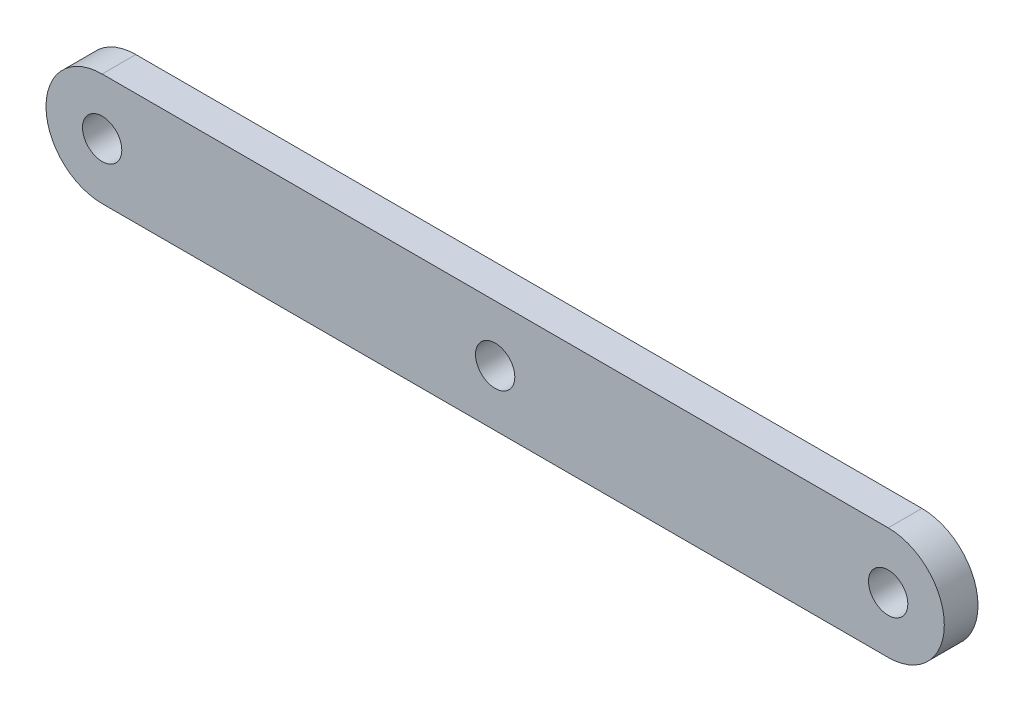
SolidWorks part; units mm, degrees
ref_plane "Front Plane" through (0, 0, 0) normal (0, 0, 1) x (1, 0, 0)
ref_plane "Top Plane" through (0, 0, 0) normal (0, 1, 0) x (1, 0, 0)
ref_plane "Right Plane" through (0, 0, 0) normal (1, 0, 0) x (0, 0, -1)
sketch "Sketch1" plane through (0, 0, 0) normal (0, 0, 1) x (1, 0, 0)
  line L0 (55, 0) -> (-55, 0) construction
  line L1 (0, 10) -> (140, 10)
  line L2 (0, 0) -> (158.2009, 0) construction
  line L3 (0, -10) -> (140, -10)
  arc A0 (0, 10) -> (0, -10) centre (0, 0) ccw
  arc A1 (140, -10) -> (140, 10) centre (140, 0) ccw
  dimension "D1" = 140
  dimension "D2" = 20
  dimension "D3" = 20
extrude "Boss-Extrude1" add sketch "Sketch1" along normal blind 6
sketch "Sketch2" plane through (0, 0, 6) normal (0, 0, 1) x (1, 0, 0)
  circle A0 centre (0, 0) radius 3.5
  circle A1 centre (140, 0) radius 3.5
  dimension "D1" = 7
  dimension "D2" = 7
extrude "Cut-Extrude1" cut sketch "Sketch2" against normal blind 95
sketch "Sketch3" plane through (0, 0, 6) normal (0, 0, 1) x (1, 0, 0)
  line L0 (0, 0) -> (140, 0) construction
  circle A0 centre (70, 0) radius 3.5
  dimension "D1" = 7
extrude "Cut-Extrude2" cut sketch "Sketch3" against normal blind 10
